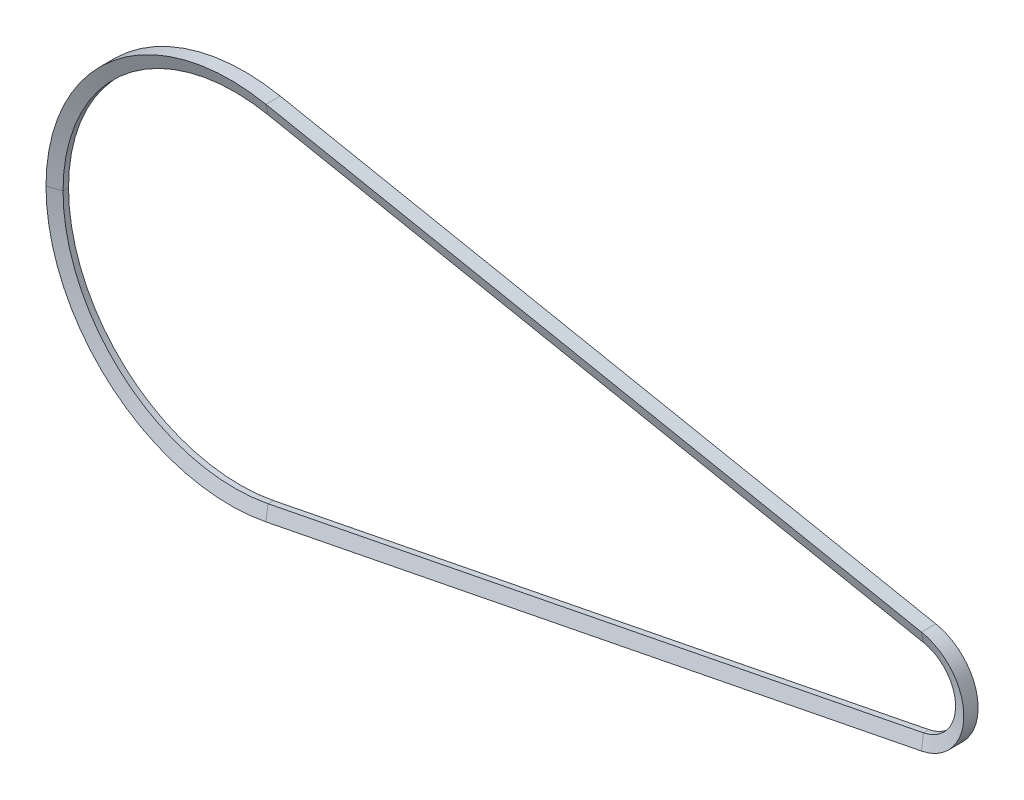
SolidWorks part; units mm, degrees
material "AISI 304"
ref_plane "Front Plane" through (0, 0, 0) normal (0, 0, 1) x (1, 0, 0)
ref_plane "Top Plane" through (0, 0, 0) normal (0, 1, 0) x (1, 0, 0)
ref_plane "Right Plane" through (0, 0, 0) normal (1, 0, 0) x (0, 0, -1)
other "Configuration Table"
sketch "Sketch1" plane through (0, 0, 0) normal (0, 0, 1) x (1, 0, 0)
  line L0 (0, 0) -> (620, 0) construction
  line L1 (30.2516, 153.3445) -> (627.0258, 35.6136)
  line L2 (627.0258, -35.6136) -> (30.2516, -153.3445)
  arc A0 (30.2516, 153.3445) -> (30.2516, -153.3445) centre (0, 0) ccw
  arc A1 (627.0258, -35.6136) -> (627.0258, 35.6136) centre (620, 0) ccw
  dimension "D1" = 312.6
  dimension "D2" = 72.6
  dimension "D3" = 620
sketch "Sketch2" plane through (0, 0, 0) normal (0, 1, 0) x (1, 0, 0)
  line L0 (-156.3, 0) -> (-156.3, -5)
  line L1 (0, 0) -> (620, 0) construction
  line L2 (-156.3, -2.5) -> (-167.8, -2.5) construction
  line L3 (-167.8, 4) -> (-167.8, -9)
  line L4 (-167.8, 4) -> (-156.3, 0)
  line L5 (-156.3, -5) -> (-167.8, -9)
  point P3 (-156.3, -2.5)
  point P11 (-167.8, -2.5)
  dimension "D1" = 156.3
  dimension "D2" = 5
  dimension "D3" = 2.5
  dimension "D4" = 13
  dimension "D5" = 11.5
sweep "Sweep1" add profiles "Sketch2" path "Sketch1"
